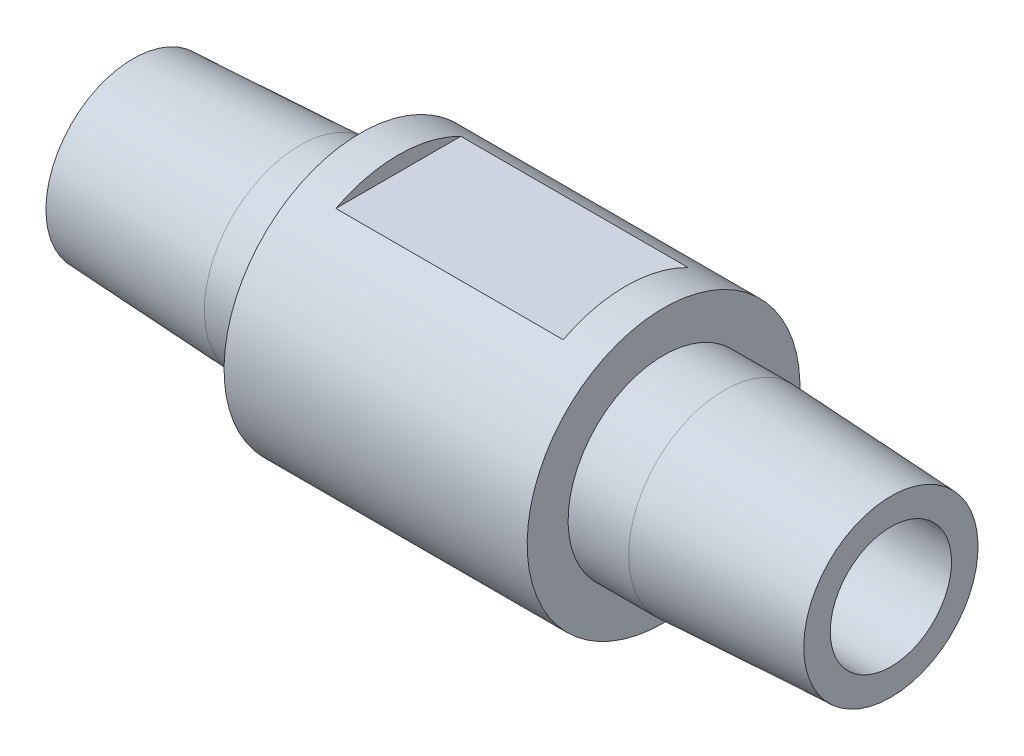
SolidWorks part; units mm, degrees
material "CuCrZr"
ref_plane "前视基准面" through (0, 0, 0) normal (0, 0, 1) x (1, 0, 0)
ref_plane "上视基准面" through (0, 0, 0) normal (0, 1, 0) x (1, 0, 0)
ref_plane "右视基准面" through (0, 0, 0) normal (1, 0, 0) x (0, 0, -1)
sketch "草图1" plane through (0, 0, 0) normal (0, 0, 1) x (1, 0, 0)
  line L0 (0, 0) -> (59, 0) construction
  line L1 (0, 4) -> (0, 5.75)
  line L2 (35, 9) -> (15, 9)
  line L3 (0, 0) -> (10, 0) construction
  line L4 (10, 0) -> (10, 0.5) construction
  line L5 (10, 0.5) -> (0, 0) construction
  line L7 (0, 5.75) -> (11, 6.3)
  line L8 (11, 6.3) -> (15, 6.3)
  line L9 (15, 6.3) -> (15, 9)
  line L10 (35, 6.3) -> (35, 9)
  line L12 (39, 6.3) -> (35, 6.3)
  line L13 (50, 5.75) -> (39, 6.3)
  line L15 (50, 4) -> (50, 5.75)
  line L16 (49, 0) -> (0, 0) construction
  line L18 (0, 0) -> (0, 5.75) construction
  line L19 (0, 4) -> (50, 4)
  line L20 (25, 4) -> (25, 17.5942) construction
  dimension "D1" = 12.6
  dimension "D2" = 18
  dimension "D3" = 8
  dimension "D4" = 11
  dimension "D5" = 50
  dimension "D6" = 4
  dimension "D7" = 0.5
  dimension "D8" = 10
revolve "旋转1" add sketch "草图1" angle 360 about L0
ref_plane "基准面1" through (25, 0, 0) normal (-1, 0, 0) x (0, 0, 1)
sketch "草图2" plane through (25, 0, 0) normal (-1, 0, 0) x (0, 0, 1)
  line L1 (-10.4529, 8) -> (10.4529, 8)
  line L2 (-10.4529, 8) -> (-10.4529, -8)
  line L3 (-10.4529, -8) -> (10.4529, -8)
  line L4 (10.4529, 8) -> (10.4529, -8)
  line L5 (0, -8) -> (0, 8) construction
  line L6 (-10.4529, 0) -> (10.4529, 0) construction
  point P0 (0, 0)
  dimension "D1" = 16
extrude "切除-拉伸1" cut sketch "草图2" against normal mid plane 15 flip side to cut
